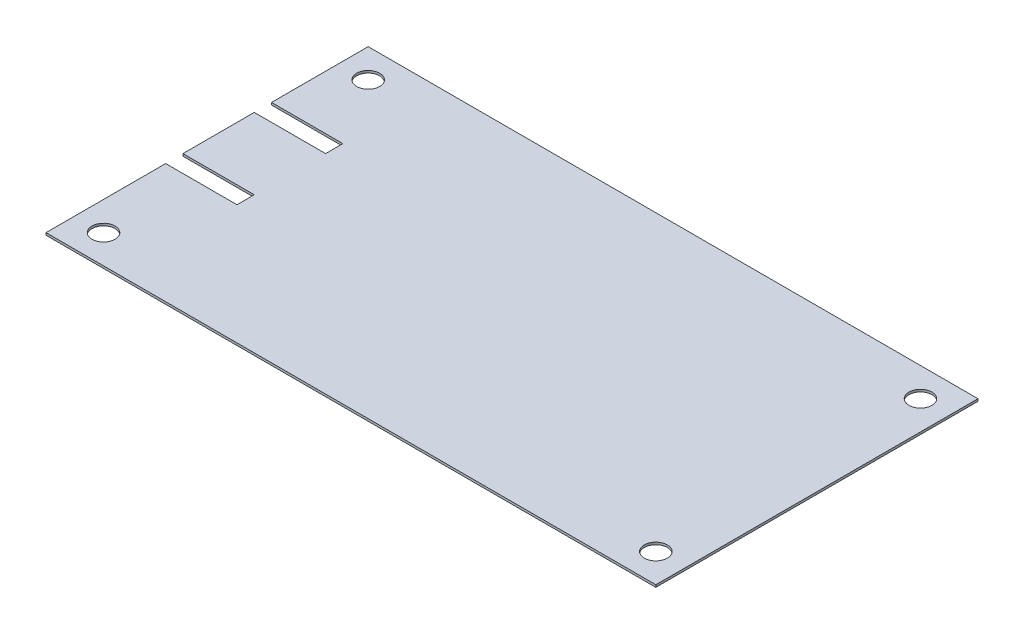
from build123d import *

# Parameters (mm, degrees)
SKETCH_1_W          = 530
SKETCH_1_H          = 280
EXTRUDE_1_DEPTH     = 2
SKETCH_2_R          = 10
CUT_EXTRUDE_1_DEPTH = 2
SKETCH_3_W          = 96.084131949
SKETCH_3_H          = 15
SKETCH_3_W_2        = 93.312729878
CUT_EXTRUDE_2_DEPTH = 10


with BuildPart() as part:
    # 草图1 → 凸台-拉伸1 (new body)
    with BuildSketch(Plane(origin=(0, 0, 0), x_dir=(1, 0, 0), z_dir=(0, 1, 0))):
        Rectangle(SKETCH_1_W, SKETCH_1_H)
    extrude(amount=EXTRUDE_1_DEPTH)

    # 草图2 → 切除-拉伸1 (cut)
    with BuildSketch(Plane(origin=(0, 2, 0), x_dir=(1, 0, 0), z_dir=(0, 1, 0))):
        with Locations(Location((-240, 115, 0), (0, 0, 270))):
            Circle(SKETCH_2_R)
        with Locations(Location((-240, -115, 0), (0, 0, 90))):
            Circle(SKETCH_2_R)
        with Locations(Location((240, -115, 0), (0, 0, 270))):
            Circle(SKETCH_2_R)
        with Locations(Location((240, 115, 0), (0, 0, 90))):
            Circle(SKETCH_2_R)
    extrude(amount=-CUT_EXTRUDE_1_DEPTH, mode=Mode.SUBTRACT)

    # 草图3 → 切除-拉伸2 (cut)
    with BuildSketch(Plane(origin=(0, 2, 0), x_dir=(1, 0, 0), z_dir=(0, 1, 0))):
        with Locations((-251.042065975, -28.5)):
            Rectangle(SKETCH_3_W, SKETCH_3_H)
        with Locations((-249.656364939, 48.5)):
            Rectangle(SKETCH_3_W_2, SKETCH_3_H)
    extrude(amount=-CUT_EXTRUDE_2_DEPTH, mode=Mode.SUBTRACT)


solid = part.part
